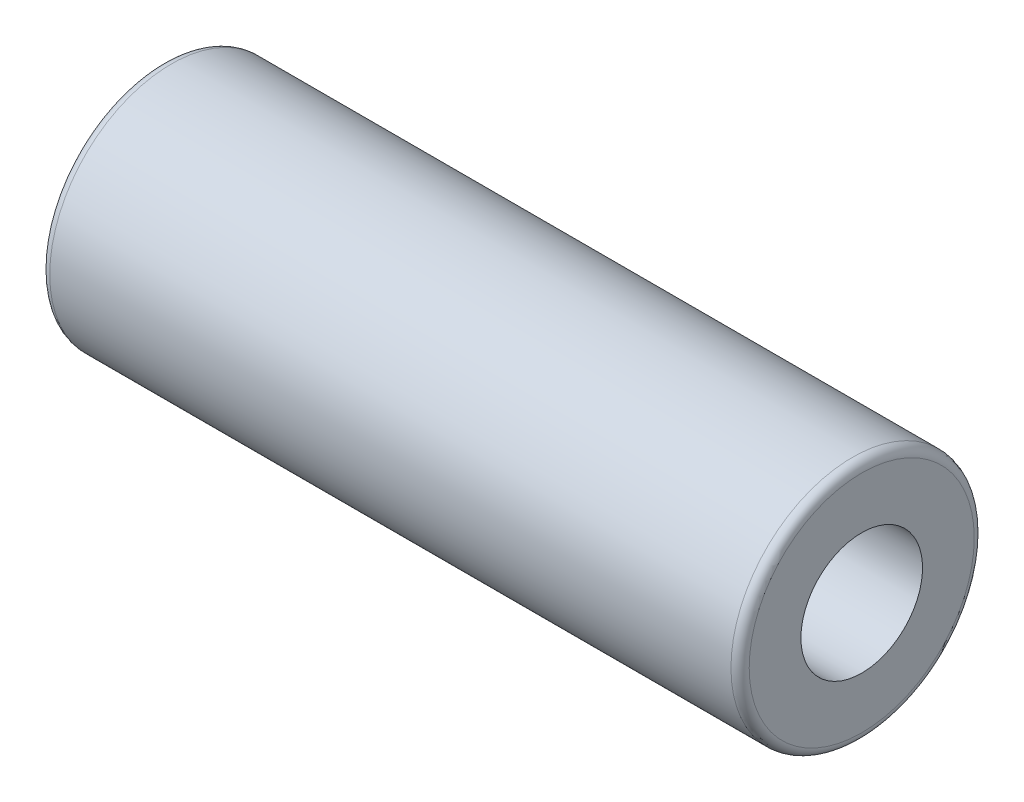
from build123d import *


with BuildPart() as part:
    # Sketch1 → Revolve1 (revolve)
    with BuildSketch(Plane.XY, mode=Mode.PRIVATE) as revolve1_sk:
        with BuildLine():
            Line((0, 2), (23, 2))
            Line((23, 2), (23, 3.7))
            ThreePointArc((23, 3.7), (22.912132034, 3.912132034), (22.7, 4))
            Line((22.7, 4), (0.3, 4))
            ThreePointArc((0.3, 4), (0.087867966, 3.912132034), (0, 3.7))
            Line((0, 3.7), (0, 2))
        make_face()
    revolve(revolve1_sk.sketch.rotate(Axis((50, 0, 0), (-1, 0, 0)), 270), axis=Axis((50, 0, 0), (-1, 0, 0)))


solid = part.part
